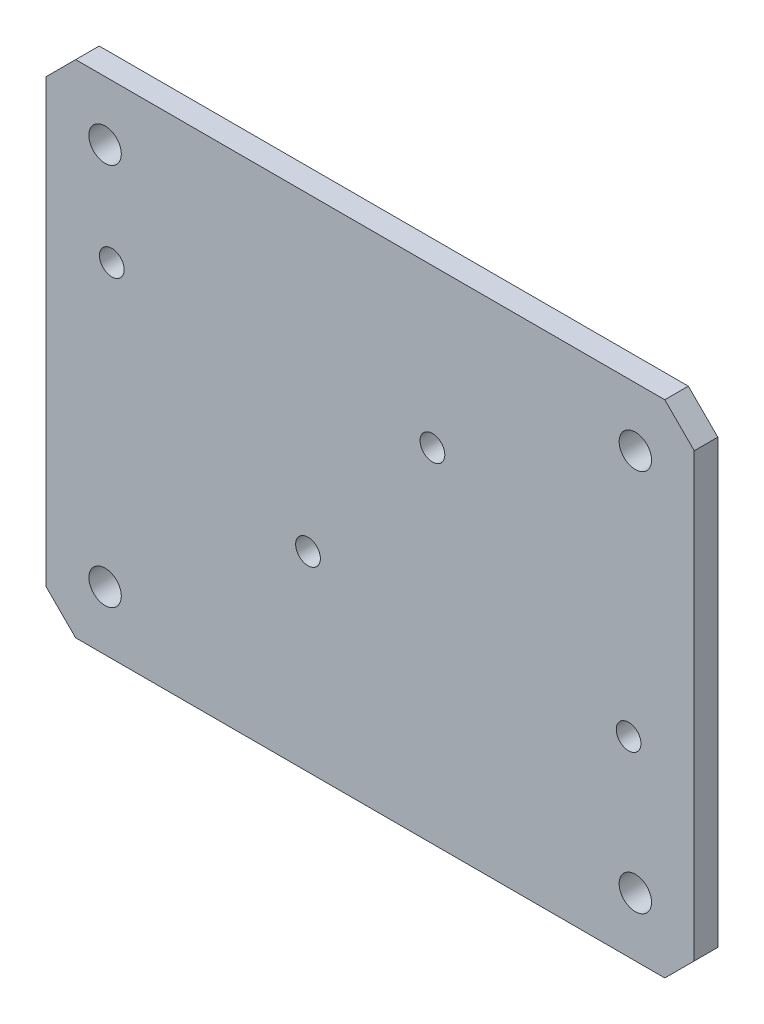
from build123d import *

# Parameters (mm, degrees)
SKETCH_1_W                  = 110
SKETCH_1_H                  = 85
EXTRUDE_1_DEPTH             = 2
CHAMFER_1_SIZE              = 5
HOLE_WIZARD_5_5_5_5_1_D     = 5.5
HOLE_WIZARD_5_5_5_5_1_DEPTH = 15.61
HOLE_WIZARD_5_5_5_5_1_TIP   = 1.58771324
HOLE_WIZARD_M5_3_D          = 4.2


with BuildPart() as part:
    # 草图1 → 凸台-拉伸1 (new, symmetric)
    with BuildSketch(Plane.XY):
        Rectangle(SKETCH_1_W, SKETCH_1_H)
    extrude(amount=EXTRUDE_1_DEPTH, both=True)

    # 倒角1
    chamfer_1_edges = [part.edges().sort_by_distance(p)[0] for p in [
        (-55, 42.5, 0),
        (55, 42.5, 0),
        (55, -42.5, 0),
        (-55, -42.5, 0),
    ]]
    chamfer(chamfer_1_edges, length=CHAMFER_1_SIZE)

    # Ø5.5 (5.5) 直径孔1
    with Locations(Plane.XY.offset(2)):
        with Locations((45, 32.5), (45, -32.5), (-45, -32.5), (-45, 32.5)):
            Hole(HOLE_WIZARD_5_5_5_5_1_D / 2, depth=HOLE_WIZARD_5_5_5_5_1_DEPTH)
            with Locations((0, 0, -(HOLE_WIZARD_5_5_5_5_1_DEPTH + HOLE_WIZARD_5_5_5_5_1_TIP / 2))):  # 120° drill point
                Cone(0, HOLE_WIZARD_5_5_5_5_1_D / 2, HOLE_WIZARD_5_5_5_5_1_TIP, mode=Mode.SUBTRACT)

    # M5 螺纹孔3 (through all)
    with Locations(Plane.XY.offset(2)):
        with Locations((-43.86, 15.732567746), (10.56, 15.732567746), (-10.56, -10.077432254), (43.86, -10.077432254)):
            Hole(HOLE_WIZARD_M5_3_D / 2)


solid = part.part
